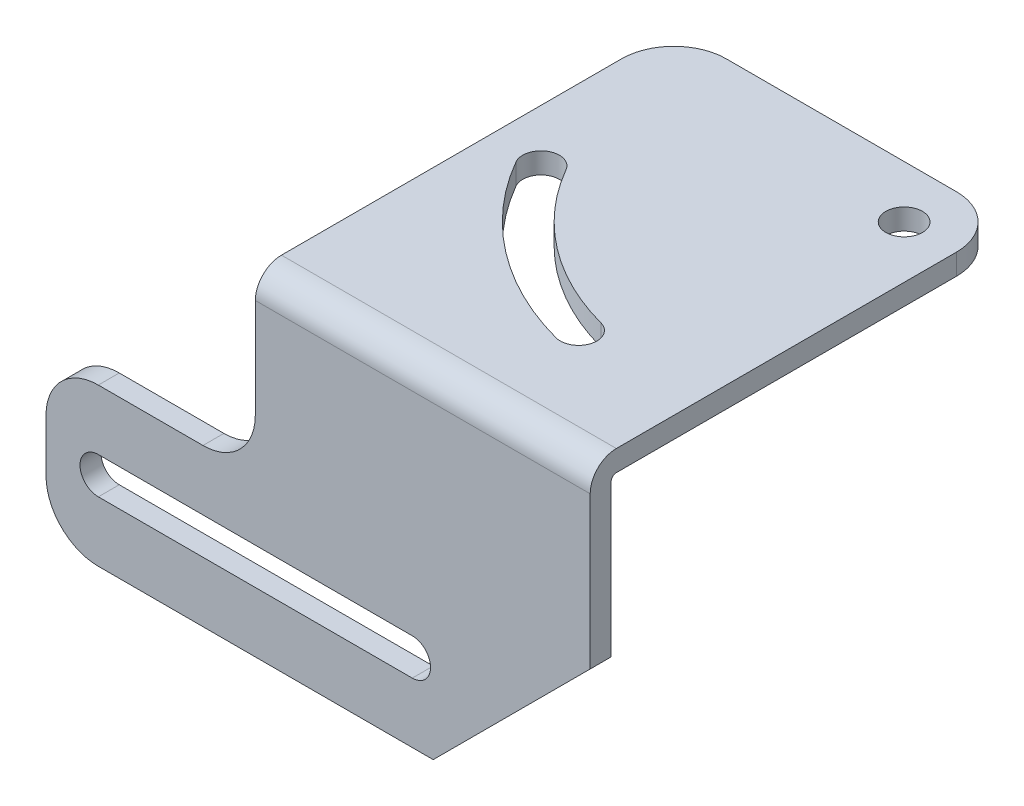
from build123d import *

# Parameters (mm, degrees)
SKETCH_1_W              = 32
SKETCH_1_H              = 40
EXTRUDE_1_DEPTH         = 32
SKETCH_2_W              = 45.589932218
SKETCH_2_H              = 35.821991612
CUT_EXTRUDE_1_DEPTH     = 72.582120673
HOLE_WIZARD_3_5_3_5_1_D = 3.5
FILLET_1_R              = 0.5
FILLET_3_R              = 2.5
CUT_EXTRUDE_3_REACH     = 69.439
SKETCH_9_W              = 2
SKETCH_9_H              = 15
EXTRUDE_2_DEPTH         = 20
CUT_EXTRUDE_4_DEPTH     = 64.780874876
CHAMFER_1_SIZE          = 15
FILLET_4_R              = 5


with BuildPart() as part:
    # 草图1 → 凸台-拉伸1 (new body)
    with BuildSketch(Plane(origin=(0, 0, 0), x_dir=(0, -1, 0), z_dir=(-1, 0, 0))):
        with Locations((24, -30)):
            Rectangle(SKETCH_1_W, SKETCH_1_H)
    extrude(amount=-EXTRUDE_1_DEPTH)

    # 草图2 → 切除-拉伸1 (cut, through all)
    with BuildSketch(Plane(origin=(32, 0, 0), x_dir=(0, 0, -1), z_dir=(1, 0, 0))):
        with Locations((34.794966109, -27.910995806)):
            Rectangle(SKETCH_2_W, SKETCH_2_H)
    extrude(amount=-CUT_EXTRUDE_1_DEPTH, mode=Mode.SUBTRACT)

    # Ø3.5 (3.5) 直径孔1 (through all)
    with Locations(Plane(origin=(0, -10, 0), x_dir=(-1, 0, 0), z_dir=(0, -1, 0))):
        with Locations((-5.002954744, 32.3), (-27, 45)):
            Hole(HOLE_WIZARD_3_5_3_5_1_D / 2)

    # 圆角1
    fillet_1_edges = [part.edges().sort_by_distance(p)[0] for p in [
        (16, -10, -12),
    ]]
    fillet(fillet_1_edges, radius=FILLET_1_R)

    # 圆角3
    fillet_3_edges = [part.edges().sort_by_distance(p)[0] for p in [
        (16, -8, -10),
    ]]
    fillet(fillet_3_edges, radius=FILLET_3_R)

    # 草图8 → 切除-拉伸3 (cut, up to next)
    with BuildSketch(Plane(origin=(0, -8, 0), x_dir=(1, 0, 0), z_dir=(0, 1, 0)), mode=Mode.PRIVATE) as cut_extrude_3_sk1:
        with BuildLine():
            ThreePointArc((3.487410287, 31.425), (10.472127202, 23.460456811), (19.973062925, 18.775113816))
            ThreePointArc((19.973062925, 18.775113816), (22.11636645, 20.012550683), (20.878929583, 22.155854208))
            ThreePointArc((20.878929583, 22.155854208), (12.602792204, 26.237193502), (6.5184992, 33.175))
            ThreePointArc((6.5184992, 33.175), (4.127954744, 33.815544457), (3.487410287, 31.425))
        make_face()
    cut_extrude_3_tool1 = extrude(cut_extrude_3_sk1.sketch, amount=-CUT_EXTRUDE_3_REACH, mode=Mode.PRIVATE) & part.part
    add(cut_extrude_3_tool1.solids().sort_by_distance((12.026611, -8, -25.486299))[0], mode=Mode.SUBTRACT)

    # 草图9 → 凸台-拉伸2 (add)
    with BuildSketch(Plane.ZY):
        with Locations((-11, -32.5)):
            Rectangle(SKETCH_9_W, SKETCH_9_H)
    extrude(amount=EXTRUDE_2_DEPTH)

    # 草图10 → 切除-拉伸4 (cut, through all)
    with BuildSketch(Plane(origin=(0, 0, -12), x_dir=(-1, 0, 0), z_dir=(0, 0, -1))):
        with BuildLine():
            Line((-15, -30.75), (15, -30.75))
            ThreePointArc((15, -30.75), (16.75, -32.5), (15, -34.25))
            Line((15, -34.25), (-15, -34.25))
            ThreePointArc((-15, -34.25), (-16.75, -32.5), (-15, -30.75))
        make_face()
    extrude(amount=-CUT_EXTRUDE_4_DEPTH, mode=Mode.SUBTRACT)

    # 倒角1
    chamfer_1_edges = [part.edges().sort_by_distance(p)[0] for p in [
        (32, -40, -11),
    ]]
    chamfer(chamfer_1_edges, length=CHAMFER_1_SIZE)

    # 圆角4
    fillet_4_edges = [part.edges().sort_by_distance(p)[0] for p in [
        (-20, -40, -11),
        (0, -25, -11),
        (-20, -25, -11),
        (0, -9, -50),
        (32, -9, -50),
    ]]
    fillet(fillet_4_edges, radius=FILLET_4_R)


solid = part.part
